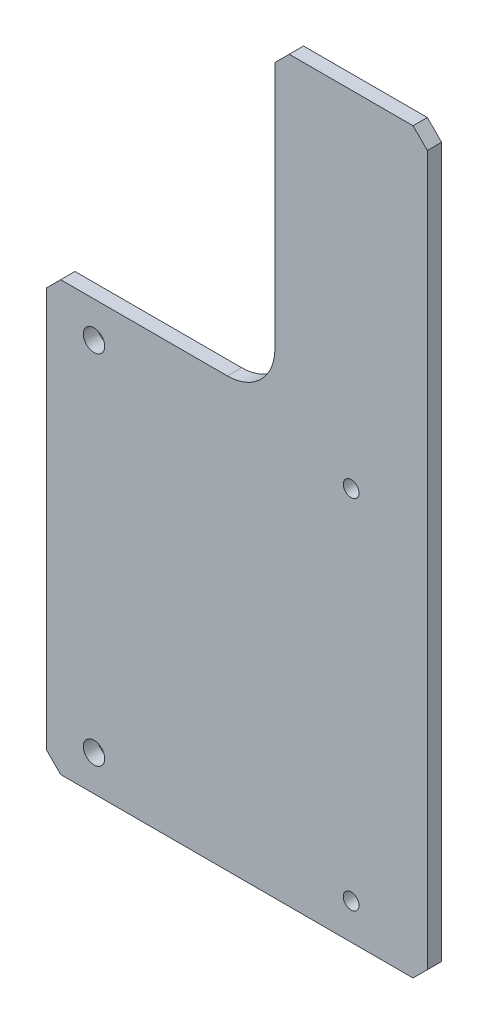
from build123d import *

# Parameters (mm, degrees)
SKETCH1_W            = 80
SKETCH1_H            = 155
BOSS_EXTRUDE1_DEPTH  = 3
M4_TAPPED_HOLE1_D    = 3.3
M4_CLEARANCE_HOLE1_D = 4.5
SKETCH8_W            = 48
SKETCH8_H            = 65
CUT_EXTRUDE1_DEPTH   = 175.453432182
CHAMFER1_SIZE        = 3
FILLET1_R            = 10


with BuildPart() as part:
    # Sketch1 → Boss-Extrude1 (new body)
    with BuildSketch(Plane.XY):
        with Locations((40, 77.5)):
            Rectangle(SKETCH1_W, SKETCH1_H)
    extrude(amount=BOSS_EXTRUDE1_DEPTH)

    # M4 Tapped Hole1 (through all)
    with Locations(Plane.XY.offset(3)):
        with Locations((64, 82.5), (64, 7.5)):
            Hole(M4_TAPPED_HOLE1_D / 2)

    # M4 Clearance Hole1 (through all)
    with Locations(Plane.XY.offset(3)):
        with Locations((10, 82.5), (10, 7.5)):
            Hole(M4_CLEARANCE_HOLE1_D / 2)

    # Sketch8 → Cut-Extrude1 (cut, through all)
    with BuildSketch(Plane.XY.offset(3)):
        with Locations((24, 122.5)):
            Rectangle(SKETCH8_W, SKETCH8_H)
    extrude(amount=-CUT_EXTRUDE1_DEPTH, mode=Mode.SUBTRACT)

    # Chamfer1
    chamfer1_edges = [part.edges().sort_by_distance(p)[0] for p in [
        (48, 155, 1.5),
        (0, 90, 1.5),
        (80, 155, 1.5),
        (80, 0, 1.5),
        (0, 0, 1.5),
    ]]
    chamfer(chamfer1_edges, length=CHAMFER1_SIZE)

    # Fillet1
    fillet1_edges = [part.edges().sort_by_distance(p)[0] for p in [
        (48, 90, 1.5),
    ]]
    fillet(fillet1_edges, radius=FILLET1_R)


solid = part.part
